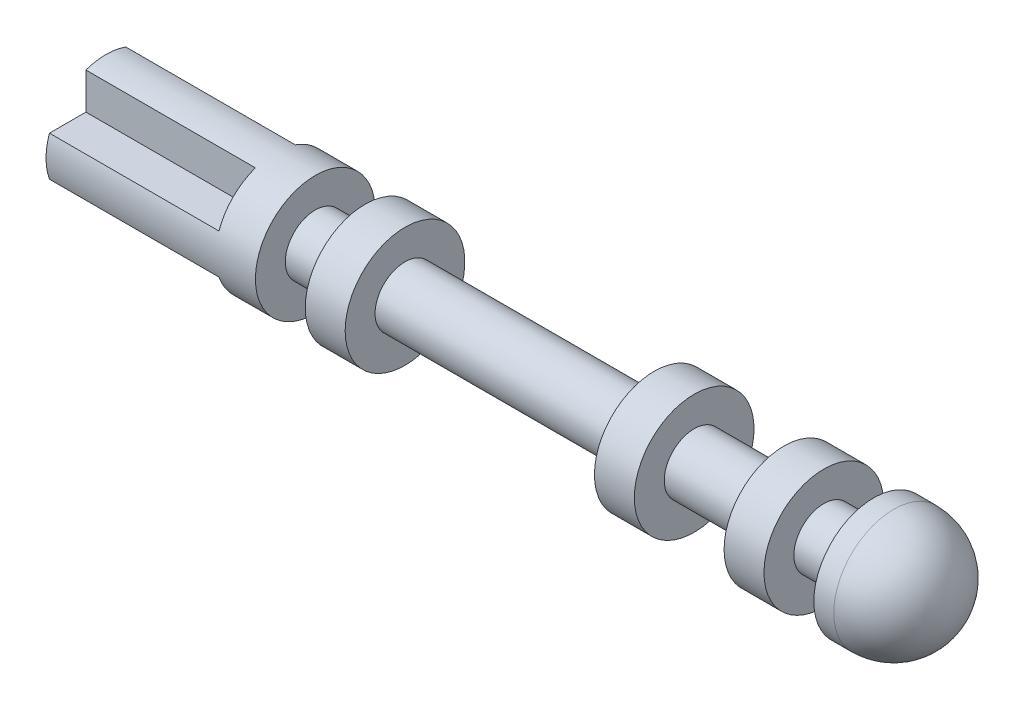
from build123d import *

# Parameters (mm, degrees)
CUT_EXTRUDE1_START = -8.5
CUT_EXTRUDE1_DEPTH = 8.5


with BuildPart() as part:
    # Sketch1 → Revolve1 (revolve)
    with BuildSketch(Plane.XY, mode=Mode.PRIVATE) as revolve1_sk:
        with BuildLine():
            Line((0, 0), (0, 3))
            Line((0, 3), (10.5, 3))
            Line((10.5, 3), (10.5, 1.5))
            Line((10.5, 1.5), (13, 1.5))
            Line((13, 1.5), (13, 3))
            Line((13, 3), (15, 3))
            Line((15, 3), (15, 1.5))
            Line((15, 1.5), (27.5, 1.5))
            Line((27.5, 1.5), (27.5, 3))
            Line((27.5, 3), (29.5, 3))
            Line((29.5, 3), (29.5, 1.5))
            Line((29.5, 1.5), (34, 1.5))
            Line((34, 1.5), (34, 3))
            Line((34, 3), (36, 3))
            Line((36, 3), (36, 1.5))
            Line((36, 1.5), (38.5, 1.5))
            Line((38.5, 1.5), (38.5, 3))
            Line((38.5, 3), (39.5, 3))
            ThreePointArc((39.5, 3), (41.621320344, 2.121320344), (42.5, 0))
            Line((42.5, 0), (0, 0))
        make_face()
    revolve(revolve1_sk.sketch.rotate(Axis((0, 0, 0), (1, 0, 0)), 90), axis=Axis((0, 0, 0), (1, 0, 0)))

    # Sketch2 → Cut-Extrude1 (cut)
    with BuildSketch(Plane.ZY.offset(CUT_EXTRUDE1_START)):
        with BuildLine():
            Line((1, 2.828427125), (1, 1))
            Line((1, 1), (2.828427125, 1))
            ThreePointArc((2.828427125, 1), (2.121320344, 2.121320344), (1, 2.828427125))
        make_face()
        with BuildLine():
            Line((2.828427125, -1), (1, -1))
            Line((1, -1), (1, -2.828427125))
            ThreePointArc((1, -2.828427125), (2.121320344, -2.121320344), (2.828427125, -1))
        make_face()
        with BuildLine():
            ThreePointArc((-1, 2.828427125), (-2.121320344, 2.121320344), (-2.828427125, 1))
            Line((-2.828427125, 1), (-1, 1))
            Line((-1, 1), (-1, 2.828427125))
        make_face()
        with BuildLine():
            Line((-1, -1), (-2.828427125, -1))
            ThreePointArc((-2.828427125, -1), (-2.121320344, -2.121320344), (-1, -2.828427125))
            Line((-1, -2.828427125), (-1, -1))
        make_face()
    extrude(amount=CUT_EXTRUDE1_DEPTH, mode=Mode.SUBTRACT)


solid = part.part
